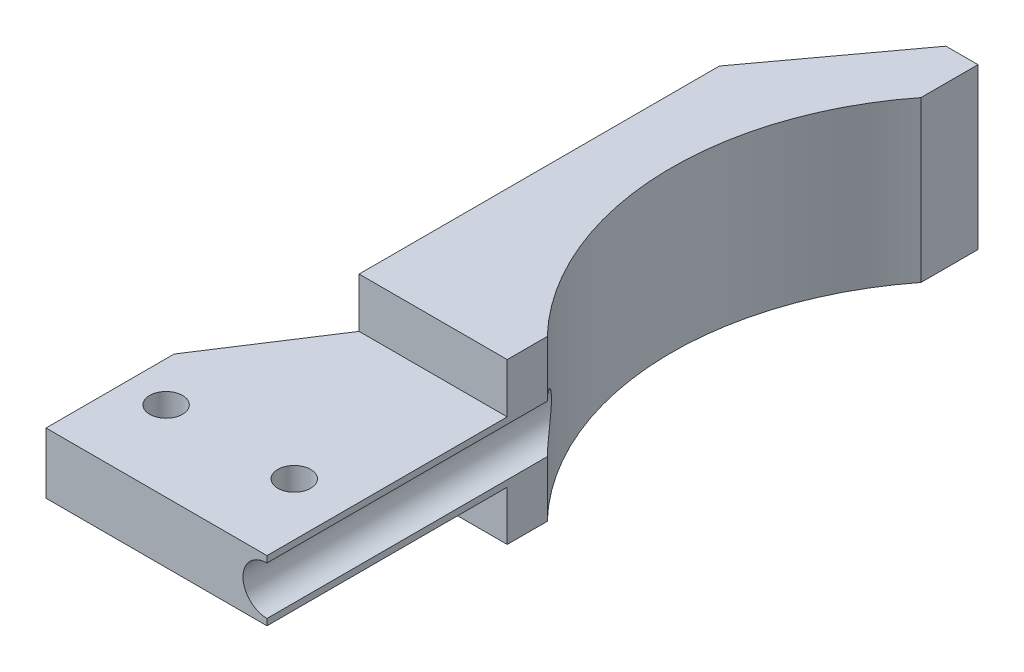
from build123d import *

# Parameters (mm, degrees)
BOSS_EXTRUDE1_DEPTH = 12.7
SKETCH1_5_R         = 2.6035
BOSS_EXTRUDE2_DEPTH = 4.826
SKETCH2_R           = 3.81
CUT_EXTRUDE1_DEPTH  = 50.038


with BuildPart() as part:
    # Sketch1 → Boss-Extrude1 (new, symmetric)
    with BuildSketch(Plane(origin=(0, 0, 0), x_dir=(1, 0, 0), z_dir=(0, 1, 0))):
        with BuildLine():
            Line((-23.495, 17.749485254), (-23.495, -39.400514746))
            Line((-23.495, -39.400514746), (0, -39.400514746))
            Line((0, -39.400514746), (0, -33.050514746))
            ThreePointArc((0, -33.050514746), (-13.273575299, -2.418042558), (-3.175, 29.402625733))
            Line((-3.175, 29.402625733), (-3.175, 38.444242963))
            Line((-3.175, 38.444242963), (-8.255, 38.444242963))
            Line((-8.255, 38.444242963), (-23.495, 17.749485254))
        make_face()
    extrude(amount=BOSS_EXTRUDE1_DEPTH, both=True)

    # Sketch1<5> → Boss-Extrude2 (add, symmetric)
    with BuildSketch(Plane(origin=(0, 0, 0), x_dir=(1, 0, 0), z_dir=(0, 1, 0))):
        Polygon((0, -39.400514746), (-23.495, -39.400514746), (-35.052, -57.180514746), (-35.052, -77.500514746), (0, -77.500514746), align=None)
        with Locations(Location((-28.702, -64.800514746, 0), (0, 0, 270))):
            Circle(SKETCH1_5_R, mode=Mode.SUBTRACT)
        with Locations(Location((-8.382, -64.800514746, 0), (0, 0, 270))):
            Circle(SKETCH1_5_R, mode=Mode.SUBTRACT)
    extrude(amount=BOSS_EXTRUDE2_DEPTH, both=True)

    # Sketch2 → Cut-Extrude1 (cut)
    with BuildSketch(Plane.XY.offset(77.500514746)):
        Circle(SKETCH2_R)
    extrude(amount=-CUT_EXTRUDE1_DEPTH, mode=Mode.SUBTRACT)


solid = part.part
